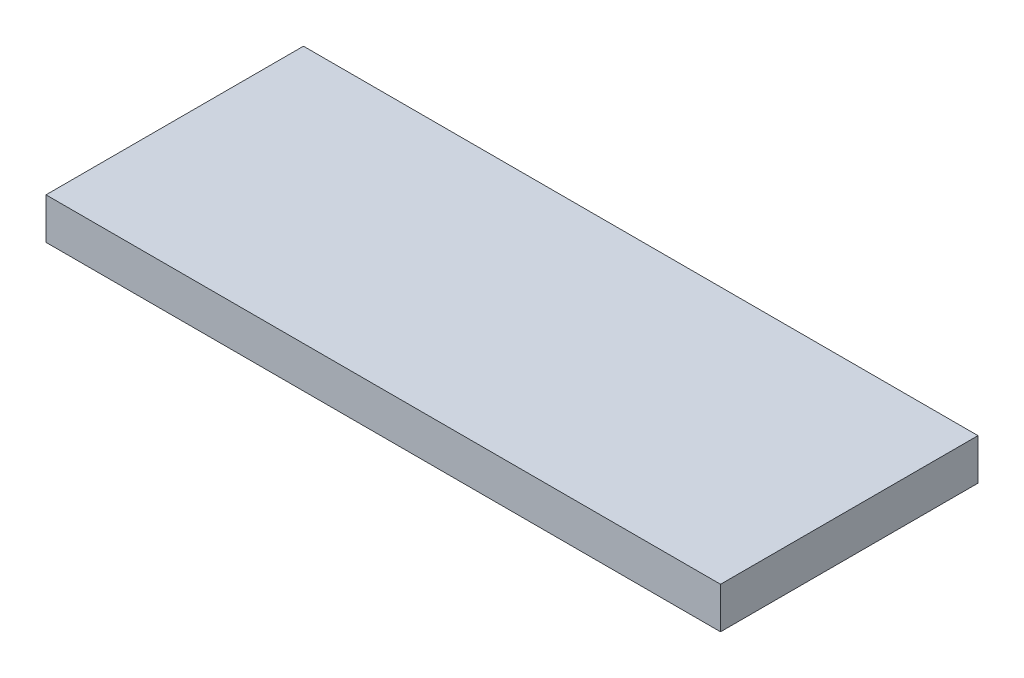
from build123d import *

# Parameters (mm, degrees)
SKETCH1_W           = 131
SKETCH1_H           = 8
BOSS_EXTRUDE1_DEPTH = 50
SKETCH2_R           = 2
CUT_EXTRUDE1_DEPTH  = 15


with BuildPart() as part:
    # Sketch1 → Boss-Extrude1 (new body)
    with BuildSketch(Plane.XY):
        with Locations((65.5, 4)):
            Rectangle(SKETCH1_W, SKETCH1_H)
    extrude(amount=BOSS_EXTRUDE1_DEPTH)

    # Sketch2 → Cut-Extrude1 (cut)
    with BuildSketch(Plane(origin=(0, 0, 0), x_dir=(-1, 0, 0), z_dir=(0, 0, -1))):
        with Locations((-122.391171487, 4)):
            Circle(SKETCH2_R)
        with Locations((-85.391171487, 4)):
            Circle(SKETCH2_R)
        with Locations((-48.391171487, 4)):
            Circle(SKETCH2_R)
        with Locations((-11.391171487, 4)):
            Circle(SKETCH2_R)
    extrude(amount=-CUT_EXTRUDE1_DEPTH, mode=Mode.SUBTRACT)


solid = part.part
